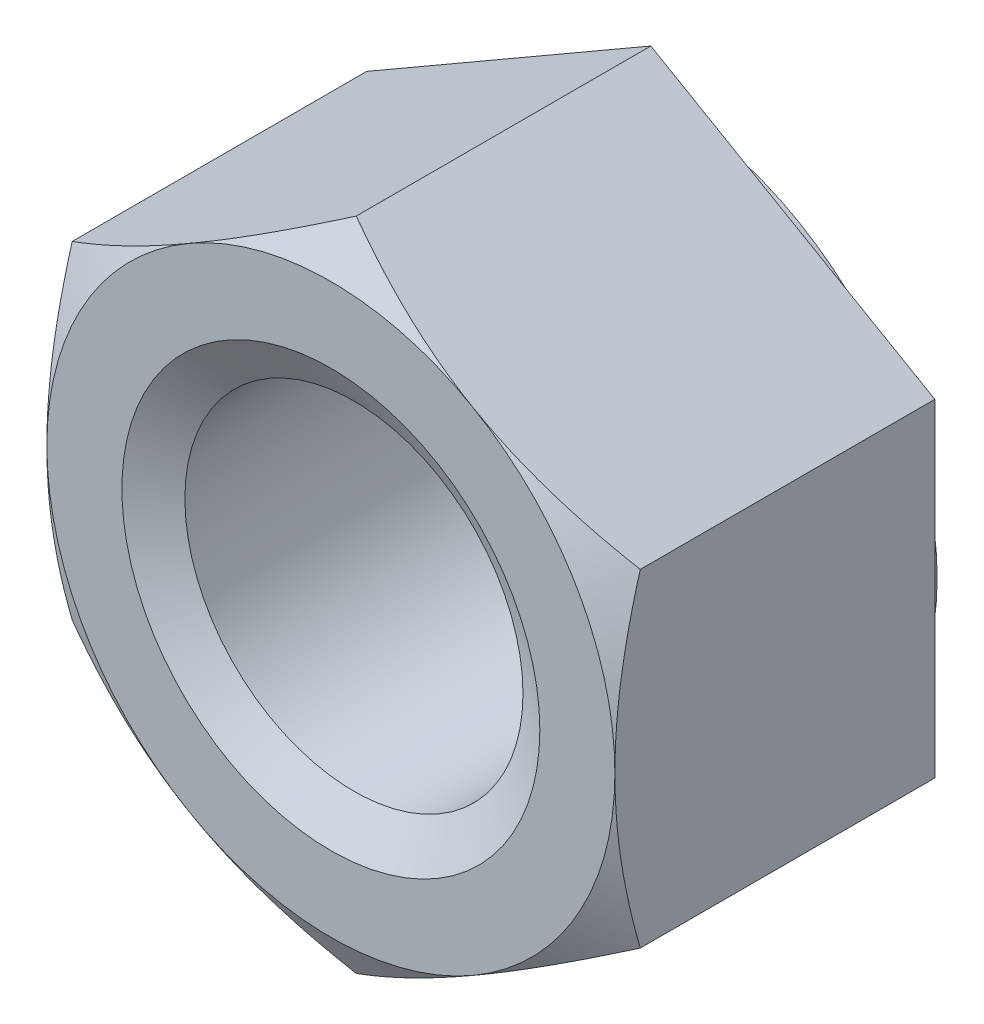
SolidWorks part; units mm, degrees
ref_plane "前视基准面" through (0, 0, 0) normal (0, 0, 1) x (1, 0, 0)
ref_plane "上视基准面" through (0, 0, 0) normal (0, 1, 0) x (1, 0, 0)
ref_plane "右视基准面" through (0, 0, 0) normal (1, 0, 0) x (0, 0, -1)
sketch "草图1" plane through (0, 0, 0) normal (1, 0, 0) x (0, 0, -1)
  line L0 (0, 25.425) -> (0, -25.425) construction
  line L1 (0, 0) -> (25.6, 0) construction
  line L2 (0, 0) -> (0, 25.425)
  line L3 (0, 25.425) -> (25.6, 25.425)
  line L4 (25.6, 25.425) -> (25.6, 0)
  line L5 (0, 15) -> (25.6, 15)
  line L6 (0, 13.1056) -> (25.6, 13.1056)
  line L7 (24.8, 25.425) -> (24.8, 0)
  line L8 (0, 23) -> (1.4001, 25.425)
  line L9 (0, 15) -> (1.0937, 13.1056)
  line L10 (0, -15) -> (1.0937, -13.1056)
  line L11 (24.8, 21.4) -> (25.6, 21.4)
  point P5 (6.2, 0)
  point P10 (22.1, 0)
  point P22 (0, 32.4)
  dimension "e" = 50.85
  dimension "m" = 25.6
  dimension "mw" = 19.4
  dimension "D" = 30
  dimension "P" = 3.5
  dimension "D81" = 26.2112
  dimension "c" = 0.8
  dimension "β" = 30
  dimension "s" = 46
  dimension "θ" = 120
  dimension "dw" = 42.8
  dimension "da" = 32.4
sketch "草图2" plane through (0, 0, 0) normal (0, 0, 1) x (1, 0, 0)
  line L1 (0, 25.425) -> (-22.0187, 12.7125)
  line L2 (-22.0187, 12.7125) -> (-22.0187, -12.7125)
  line L3 (-22.0187, -12.7125) -> (0, -25.425)
  line L4 (0, -25.425) -> (22.0187, -12.7125)
  line L5 (22.0187, -12.7125) -> (22.0187, 12.7125)
  line L6 (22.0187, 12.7125) -> (0, 25.425)
  circle A0 centre (0, 0) radius 22.0187 construction
  circle A1 centre (0, 0) radius 13.1056
sketch "草图3" plane through (0, 0, 0) normal (0, 0, 1) x (1, 0, 0)
  line L0 (0, 25.425) -> (-22.0187, 12.7125) construction
  line L1 (22.0187, 12.7125) -> (0, 25.425) construction
  line L2 (22.0187, -12.7125) -> (22.0187, 12.7125) construction
  line L3 (0, -25.425) -> (22.0187, -12.7125) construction
  line L4 (-22.0187, -12.7125) -> (0, -25.425) construction
  line L5 (-22.0187, 12.7125) -> (-22.0187, -12.7125) construction
  line L6 (0, 25.425) -> (-22.0187, 12.7125)
  line L7 (22.0187, 12.7125) -> (0, 25.425)
  line L8 (22.0187, -12.7125) -> (22.0187, 12.7125)
  line L9 (0, -25.425) -> (22.0187, -12.7125)
  line L10 (-22.0187, -12.7125) -> (0, -25.425)
  line L11 (-22.0187, 12.7125) -> (-22.0187, -12.7125)
  circle A0 centre (0, 0) radius 13.1056 construction
  circle A1 centre (0, 0) radius 13.1056
extrude "凸台-拉伸1" add sketch "草图3" against normal up to vertex (25.6 mm away) up to point (0, 0, -25.6)
cosmetic thread "装饰螺纹线1" parameters "D2"=30
sketch "草图4" plane through (0, 0, 0) normal (1, 0, 0) x (0, 0, -1)
  line L1 (0, 16.2) -> (1.7865, 13.1056)
  line L2 (0, 0) -> (25.6, 0) construction
  line L3 (0, 0) -> (25.6, 0) construction
  line L4 (12.8, 0) -> (12.8, 25.425) construction
  line L5 (0, 25.425) -> (25.6, 25.425) construction
  line L6 (1.7865, 13.1056) -> (1.7865, 0)
  line L7 (1.7865, 0) -> (0, 0)
  line L8 (0, 0) -> (0, 16.2)
  line L9 (25.6, 0) -> (25.6, 16.2)
  line L10 (23.8135, 0) -> (25.6, 0)
  line L11 (23.8135, 13.1056) -> (23.8135, 0)
  line L12 (25.6, 16.2) -> (23.8135, 13.1056)
  line L16 (0, 15) -> (1.0937, 13.1056) construction
  line L17 (0, 13.1056) -> (25.6, 13.1056) construction
  dimension "D1" = 32.4
revolve "切除-旋转1" cut sketch "草图4" angle 360 mid plane about L3
sketch "草图5" plane through (0, 0, 0) normal (0, 0, 1) x (1, 0, 0)
  circle A0 centre (0, 0) radius 22.0187
  circle A1 centre (0, 0) radius 38.1375
  circle A2 centre (0, 0) radius 22.0187 construction
  dimension "D1" = 76.275
extrude "切除-拉伸1" cut sketch "草图5" against normal blind 5.12 draft 60
sketch "草图7" plane through (0, 0, -25.6) normal (0, 0, -1) x (-1, 0, 0)
  circle A1 centre (0, 0) radius 38.1375
  circle A2 centre (0, 0) radius 38.1375
  circle A3 centre (0, 0) radius 22.0187
  circle A4 centre (0, 0) radius 22.0187
  dimension "D1" = 0
  dimension "D2" = 0
extrude "切除-拉伸2" [suppressed] cut sketch "草图7" against normal blind 5.12 draft 60
sketch "草图6" plane through (0, 0, 0) normal (1, 0, 0) x (0, 0, -1)
  line L0 (25.6, 21.4) -> (24.8, 21.4)
  line L1 (24.8, 21.4) -> (24.8, 25.425)
  line L2 (24.8, 25.425) -> (25.6, 25.425)
  line L3 (25.6, 25.425) -> (25.6, 21.4)
  line L4 (0, 0) -> (25.6, 0) construction
  line L5 (0, 0) -> (25.6, 0) construction
revolve "切除-旋转2" cut sketch "草图6" angle 360 mid plane about L5
